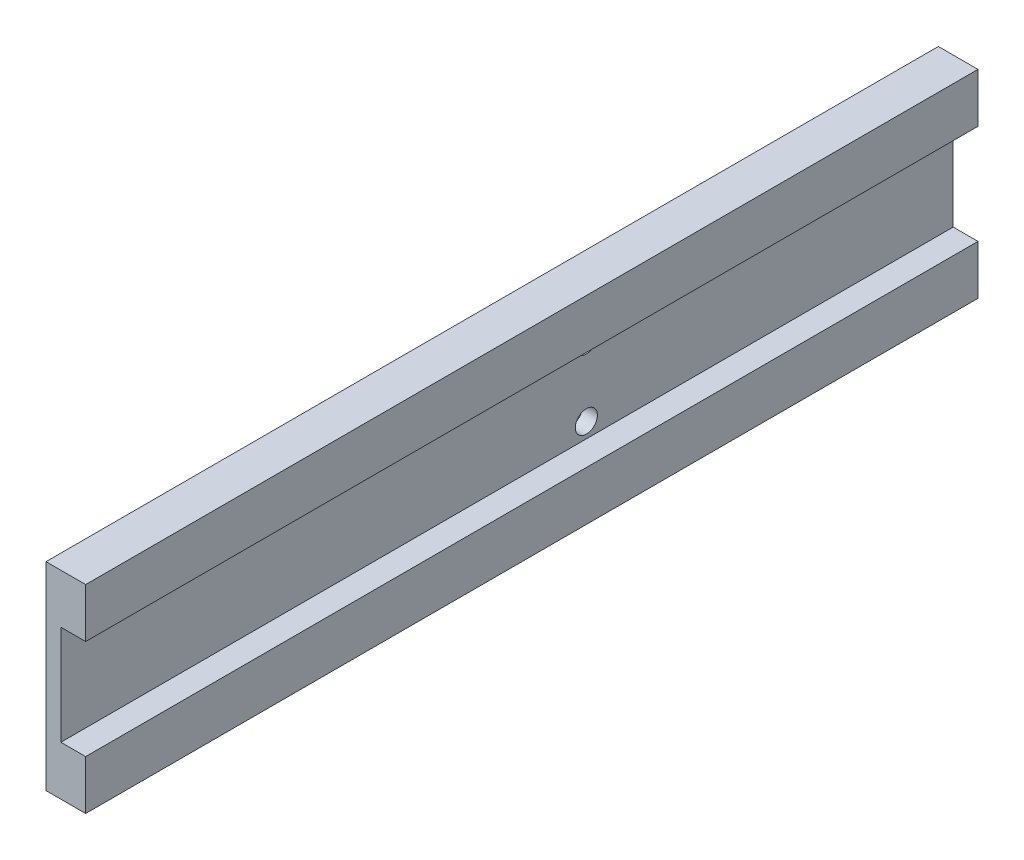
from build123d import *

# Parameters (mm, degrees)
BOSS_EXTRUDE1_DEPTH  = 900
F_1_8_TAPPED_HOLE1_D = 22.225


with BuildPart() as part:
    # Sketch1 → Boss-Extrude1 (new body)
    with BuildSketch(Plane.XY):
        Polygon((0, 0), (0, 200), (40, 200), (40, 150.25), (15, 150.25), (15, 49.75), (40, 49.75), (40, 0), align=None)
    extrude(amount=BOSS_EXTRUDE1_DEPTH)

    # 1-8 Tapped Hole1 (through all)
    with Locations(Plane(origin=(15, 135, 370), x_dir=(0, 1, 0), z_dir=(1, 0, 0))):
        with Locations((0, 0), (-70, 0)):
            Hole(F_1_8_TAPPED_HOLE1_D / 2)


solid = part.part
